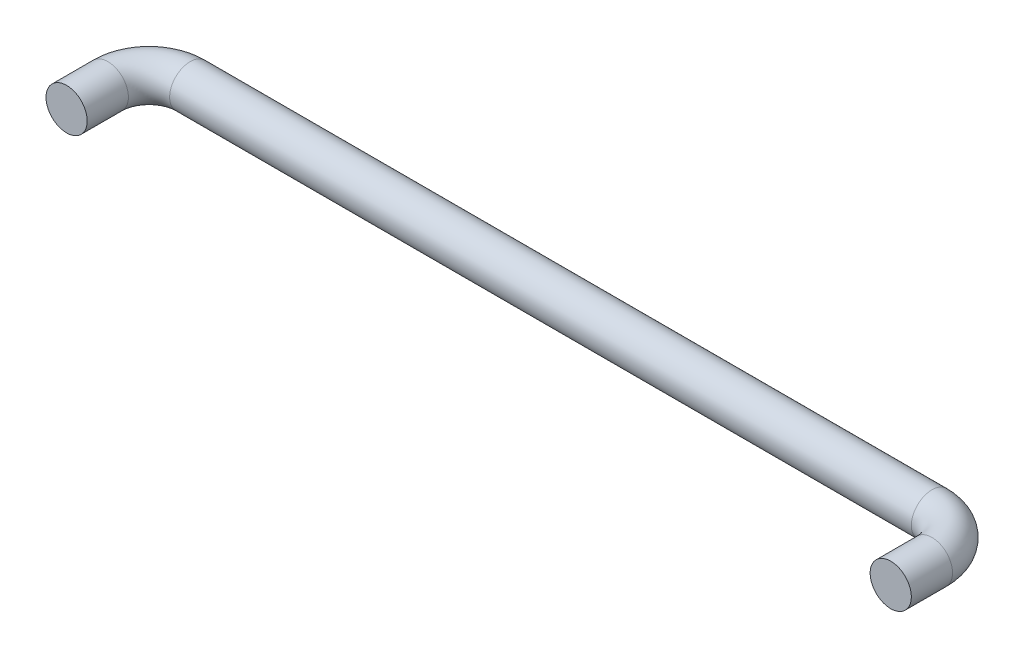
from build123d import *

# Parameters (mm, degrees)
SWEEP1_PROFILE_R = 2.5


with BuildPart() as part:
    # Sweep1: sweep along a path in Sketch1
    with BuildLine(Plane(origin=(0, 0, 0), x_dir=(1, 0, 0), z_dir=(0, 1, 0))) as sweep1_path:
        Line((0, -10), (0, -5))
        ThreePointArc((0, -5), (1.464466094, -1.464466094), (5, 0))
        Line((5, 0), (95, 0))
        ThreePointArc((95, 0), (98.535533906, -1.464466094), (100, -5))
        Line((100, -5), (100, -10))
    # Sweep1 profile (on start of the path) → Sweep1 (sweep)
    with BuildSketch(Plane(origin=(0, 0, 10), x_dir=(-1, 0, 0), z_dir=(0, 0, -1))):
        Circle(SWEEP1_PROFILE_R)
    sweep(path=sweep1_path.line)


solid = part.part
